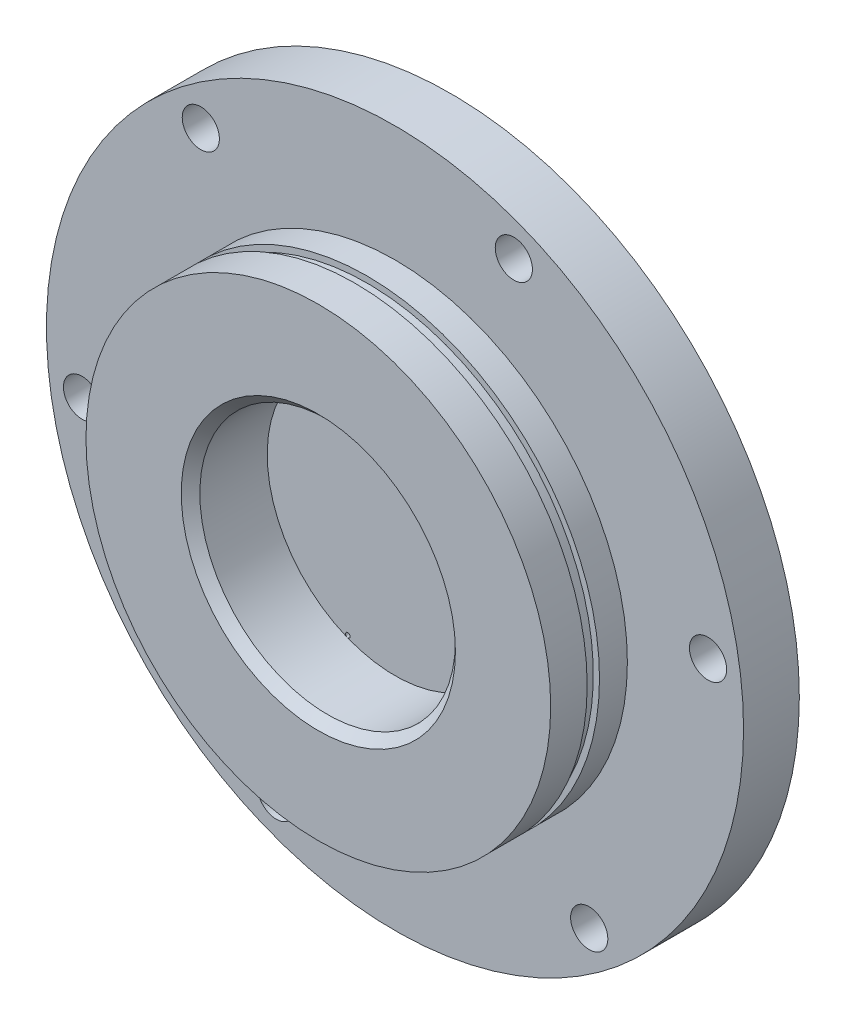
SolidWorks part; units mm, degrees
ref_plane "Front Plane" through (0, 0, 0) normal (0, 0, 1) x (1, 0, 0)
ref_plane "Top Plane" through (0, 0, 0) normal (0, 1, 0) x (1, 0, 0)
ref_plane "Right Plane" through (0, 0, 0) normal (1, 0, 0) x (0, 0, -1)
other "Configuration Table"
sketch "Sketch1" plane through (0, 0, 0) normal (0, 0, 1) x (1, 0, 0)
  circle A0 centre (0, 0) radius 75
  dimension "D1" = 150
extrude "Boss-Extrude1" add sketch "Sketch1" along normal blind 12
sketch "Sketch2" plane through (0, 0, 0) normal (0, 0, 1) x (1, 0, 0)
  circle A0 centre (0, 0) radius 50
  circle A1 centre (0, 0) radius 27.5
  dimension "D1" = 100
  dimension "D2" = 55
extrude "Boss-Extrude2" add sketch "Sketch2" along normal blind 28.5
sketch "Sketch3" plane through (0, 0, 0) normal (0, 0, -1) x (-1, 0, 0)
  circle A0 centre (0, 0) radius 50
  circle A1 centre (0, 0) radius 48.675
  dimension "D1" = 97.35
  dimension "D2" = 100
extrude "Cut-Extrude1" cut sketch "Sketch3" against normal blind 2.65 from offset 18 offset against normal yes
chamfer "Chamfer1" distance 2 angle 45 1 edges at (27.5, 0, 28.5)
sketch "Sketch7" plane through (0, 0, 0) normal (0, 0, -1) x (-1, 0, 0)
  circle A0 centre (-25.5647, 63.0115) radius 4
  circle A1 centre (41.7872, 53.6454) radius 4
  circle A2 centre (67.3519, -9.3661) radius 4
  circle A3 centre (25.5647, -63.0115) radius 4
  circle A4 centre (-41.7872, -53.6454) radius 4
  circle A5 centre (-67.3519, 9.3661) radius 4
  point P16 (0, 0)
  dimension "D1" = 8
  dimension "D2" = 68
  dimension "D3" = 6
extrude "Cut-Extrude2" cut sketch "Sketch7" against normal through all
cosmetic thread "Cosmetic Thread1" parameters "D2"=9
cosmetic thread "Cosmetic Thread2" parameters "D2"=9
cosmetic thread "Cosmetic Thread3" parameters "D2"=9
cosmetic thread "Cosmetic Thread4" parameters "D2"=9
cosmetic thread "Cosmetic Thread5" parameters "D2"=9
cosmetic thread "Cosmetic Thread6" parameters "D2"=9
sketch "Sketch10" plane through (0, 0, 0) normal (0, 0, -1) x (-1, 0, 0)
  line L0 (0, 0) -> (25.5647, -63.0115) construction
  circle A0 centre (10.1507, -25.0193) radius 2.5
  dimension "D1" = 5
  dimension "D2" = 27
extrude "Cut-Extrude3" cut sketch "Sketch10" against normal blind 7
sketch "Sketch12" plane through (0, 0, 7) normal (0, 0, -1) x (-1, 0, 0)
  circle A0 centre (10.1507, -25.0193) radius 0.5
  dimension "D1" = 1
extrude "Cut-Extrude8" cut sketch "Sketch12" against normal through all
